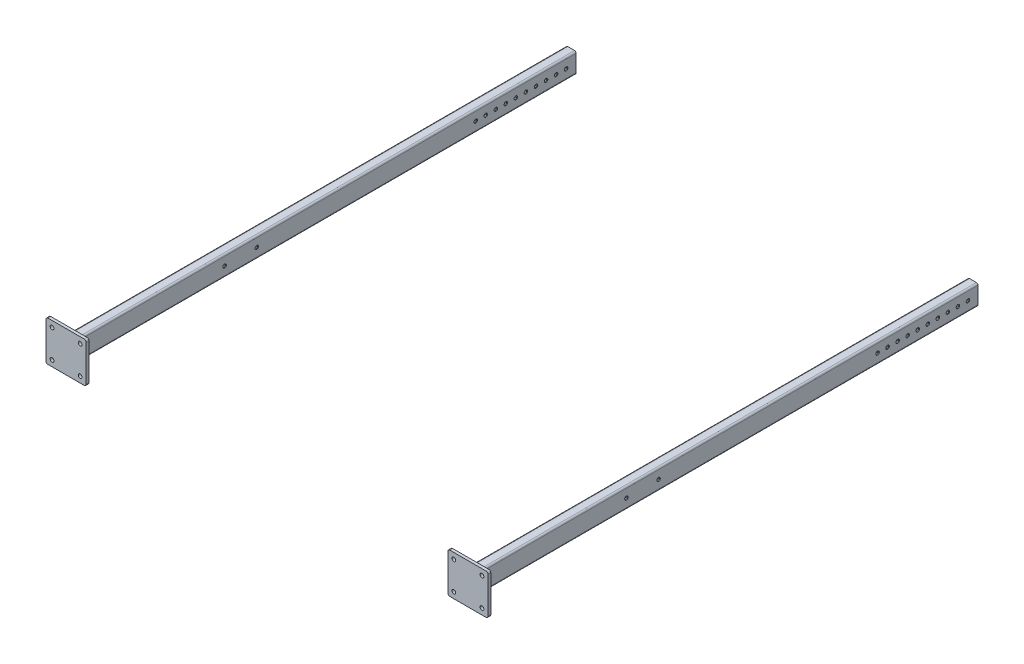
from build123d import *

# Parameters (mm, degrees)
GB_6728_1986_RECTANGULAR_HOLLOW_SECTION_DEPTH = 2500
GB_6728_1986_RECTANGULAR_HOLLOW_SECT_2_DEPTH  = 2500
SKETCH5_W                                     = 200
SKETCH5_H                                     = 200
BOSS_EXTRUDE1_DEPTH                           = 14
FILLET1_R                                     = 10
SKETCH9_W                                     = 9.5
SKETCH9_H                                     = 14
M16_CLEARANCE_HOLE1_AT_2_COUNT                = 2
M16_CLEARANCE_HOLE1_AT_2_PITCH                = 140
M16_CLEARANCE_HOLE1_AT_3_COUNT                = 2
M16_CLEARANCE_HOLE1_AT_3_PITCH                = 197.989898732
M16_CLEARANCE_HOLE1_AT_4_COUNT                = 2
M16_CLEARANCE_HOLE1_AT_4_PITCH                = 140
SKETCH14_W                                    = 8.75
SKETCH14_H                                    = 2125
LPATTERN1_COUNT                               = 10
LPATTERN1_PITCH                               = 50
SKETCH16_W                                    = 8.75
SKETCH16_H                                    = 2125
M16_CLEARANCE_HOLE4_AT_2_COUNT                = 2
M16_CLEARANCE_HOLE4_AT_2_PITCH                = 160


with BuildPart() as part:
    # Sketch12 → Gb／6728-1986 rectangular hollow section 100 X 50 X 4 (1) (new body)
    with BuildSketch(Plane(origin=(-1000, 0, 0), x_dir=(1, 0, 0), z_dir=(0, 0, -1))):
        with BuildLine():
            Line((-17, -50), (17, -50))
            ThreePointArc((17, -50), (22.656854249, -47.656854249), (25, -42))
            Line((25, -42), (25, 42))
            ThreePointArc((25, 42), (22.656854249, 47.656854249), (17, 50))
            Line((17, 50), (-17, 50))
            ThreePointArc((-17, 50), (-22.656854249, 47.656854249), (-25, 42))
            Line((-25, 42), (-25, -42))
            ThreePointArc((-25, -42), (-22.656854249, -47.656854249), (-17, -50))
        make_face()
        with BuildLine():
            Line((-17, -46), (17, -46))
            ThreePointArc((17, -46), (19.828427125, -44.828427125), (21, -42))
            Line((21, -42), (21, 42))
            ThreePointArc((21, 42), (19.828427125, 44.828427125), (17, 46))
            Line((17, 46), (-17, 46))
            ThreePointArc((-17, 46), (-19.828427125, 44.828427125), (-21, 42))
            Line((-21, 42), (-21, -42))
            ThreePointArc((-21, -42), (-19.828427125, -44.828427125), (-17, -46))
        make_face(mode=Mode.SUBTRACT)
    extrude(amount=GB_6728_1986_RECTANGULAR_HOLLOW_SECTION_DEPTH)


with BuildPart() as body_2:
    # Sketch12 on segment 2 (carried to segment 2) → Gb_6728-1986 rectangular hollow sect 2 (new body)
    with BuildSketch(Plane(origin=(1000, 0, 0), x_dir=(1, 0, 0), z_dir=(0, 0, -1))):
        with BuildLine():
            Line((-17, -50), (17, -50))
            ThreePointArc((17, -50), (22.656854249, -47.656854249), (25, -42))
            Line((25, -42), (25, 42))
            ThreePointArc((25, 42), (22.656854249, 47.656854249), (17, 50))
            Line((17, 50), (-17, 50))
            ThreePointArc((-17, 50), (-22.656854249, 47.656854249), (-25, 42))
            Line((-25, 42), (-25, -42))
            ThreePointArc((-25, -42), (-22.656854249, -47.656854249), (-17, -50))
        make_face()
        with BuildLine():
            Line((-17, -46), (17, -46))
            ThreePointArc((17, -46), (19.828427125, -44.828427125), (21, -42))
            Line((21, -42), (21, 42))
            ThreePointArc((21, 42), (19.828427125, 44.828427125), (17, 46))
            Line((17, 46), (-17, 46))
            ThreePointArc((-17, 46), (-19.828427125, 44.828427125), (-21, 42))
            Line((-21, 42), (-21, -42))
            ThreePointArc((-21, -42), (-19.828427125, -44.828427125), (-17, -46))
        make_face(mode=Mode.SUBTRACT)
    extrude(amount=GB_6728_1986_RECTANGULAR_HOLLOW_SECT_2_DEPTH)


with BuildPart() as body_3:
    # Sketch5 → Boss-Extrude1 (new body)
    with BuildSketch(Plane.XY):
        with Locations((-1000, 0)):
            Rectangle(SKETCH5_W, SKETCH5_H)
    extrude(amount=BOSS_EXTRUDE1_DEPTH)

    # Fillet1
    fillet1_edges = [body_3.edges().sort_by_distance(p)[0] for p in [
        (-900, -100, 7),
        (-1100, -100, 7),
        (-1100, 100, 7),
        (-900, 100, 7),
    ]]
    fillet(fillet1_edges, radius=FILLET1_R)

    # Sketch9 → M16 Clearance Hole1 (revolve, cut)
    with BuildSketch(Plane(origin=(-1070, 70, 0), x_dir=(0, 1, 0), z_dir=(1, 0, 0))):
        with Locations((4.75, 7)):
            Rectangle(SKETCH9_W, SKETCH9_H)
    m16_clearance_hole1 = revolve(axis=Axis((-1070, 70, -6.35), (0, 0, 1)), mode=Mode.SUBTRACT)

    # M16 Clearance Hole1 at 2: M16 Clearance Hole1 ×2
    with Locations(*[(0, -i * M16_CLEARANCE_HOLE1_AT_2_PITCH, 0) for i in range(1, M16_CLEARANCE_HOLE1_AT_2_COUNT)]):
        add(m16_clearance_hole1, mode=Mode.SUBTRACT)

    # M16 Clearance Hole1 at 3: M16 Clearance Hole1 ×2
    with Locations(*[Vector(0.7071067811865475, -0.7071067811865477, 0) * (i * M16_CLEARANCE_HOLE1_AT_3_PITCH) for i in range(1, M16_CLEARANCE_HOLE1_AT_3_COUNT)]):
        add(m16_clearance_hole1, mode=Mode.SUBTRACT)

    # M16 Clearance Hole1 at 4: M16 Clearance Hole1 ×2
    with Locations(*[(i * M16_CLEARANCE_HOLE1_AT_4_PITCH, 0, 0) for i in range(1, M16_CLEARANCE_HOLE1_AT_4_COUNT)]):
        add(m16_clearance_hole1, mode=Mode.SUBTRACT)


with BuildPart() as body_4:
    # Mirror1: mirrored copy
    add(body_3.part.mirror(Plane.ZY))


with BuildPart() as m16_clearance_hole3_tool:
    # Sketch14 → M16 Clearance Hole3 (revolve)
    with BuildSketch(Plane(origin=(1025, 0, -2450), x_dir=(0, 0, -1), z_dir=(0, 1, 0))):
        with Locations((4.375, 1062.5)):
            Rectangle(SKETCH14_W, SKETCH14_H)
    m16_clearance_hole3 = revolve(axis=Axis((1031.35, 0, -2450), (-1, 0, 0)))


with BuildPart() as part_1:
    add(part.part)

    # M16 Clearance Hole3: cut by m16_clearance_hole3_tool
    add(m16_clearance_hole3_tool.part, mode=Mode.SUBTRACT)


with BuildPart() as body_2_1:
    add(body_2.part)

    # M16 Clearance Hole3: cut by m16_clearance_hole3_tool
    add(m16_clearance_hole3_tool.part, mode=Mode.SUBTRACT)


with BuildPart() as lpattern1_tool:
    # LPattern1: M16 Clearance Hole3 ×10
    with Locations(*[(0, 0, i * LPATTERN1_PITCH) for i in range(1, LPATTERN1_COUNT)]):
        add(m16_clearance_hole3)


with BuildPart() as part_2:
    add(part_1.part)

    # LPattern1: cut by lpattern1_tool
    add(lpattern1_tool.part, mode=Mode.SUBTRACT)


with BuildPart() as body_2_2:
    add(body_2_1.part)

    # LPattern1: cut by lpattern1_tool
    add(lpattern1_tool.part, mode=Mode.SUBTRACT)


with BuildPart() as m16_clearance_hole4_tool:
    # Sketch16 → M16 Clearance Hole4 (revolve)
    with BuildSketch(Plane(origin=(-1025, 0, -750), x_dir=(0, 0, 1), z_dir=(0, 1, 0))):
        with Locations((4.375, 1062.5)):
            Rectangle(SKETCH16_W, SKETCH16_H)
    m16_clearance_hole4 = revolve(axis=Axis((-1031.35, 0, -750), (1, 0, 0)))


with BuildPart() as part_3:
    add(part_2.part)

    # M16 Clearance Hole4: cut by m16_clearance_hole4_tool
    add(m16_clearance_hole4_tool.part, mode=Mode.SUBTRACT)


with BuildPart() as body_2_3:
    add(body_2_2.part)

    # M16 Clearance Hole4: cut by m16_clearance_hole4_tool
    add(m16_clearance_hole4_tool.part, mode=Mode.SUBTRACT)


with BuildPart() as m16_clearance_hole4_at_2_tool:
    # M16 Clearance Hole4 at 2: M16 Clearance Hole4 ×2
    with Locations(*[(0, 0, -i * M16_CLEARANCE_HOLE4_AT_2_PITCH) for i in range(1, M16_CLEARANCE_HOLE4_AT_2_COUNT)]):
        add(m16_clearance_hole4)


with BuildPart() as part_4:
    add(part_3.part)

    # M16 Clearance Hole4 at 2: cut by m16_clearance_hole4_at_2_tool
    add(m16_clearance_hole4_at_2_tool.part, mode=Mode.SUBTRACT)


with BuildPart() as body_2_4:
    add(body_2_3.part)

    # M16 Clearance Hole4 at 2: cut by m16_clearance_hole4_at_2_tool
    add(m16_clearance_hole4_at_2_tool.part, mode=Mode.SUBTRACT)


solid = Compound([body_3.part, body_4.part, part_4.part, body_2_4.part])
